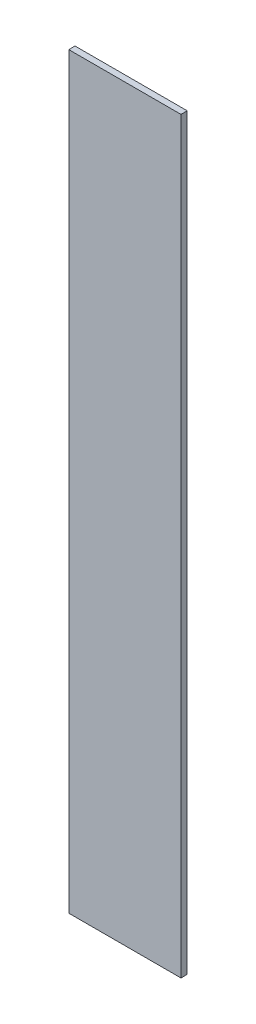
from build123d import *

# Parameters (mm, degrees)
SKETCH_1_W      = 90
SKETCH_1_H      = 600
EXTRUDE_1_DEPTH = 3
SKETCH_2_W      = 90
SKETCH_2_H      = 600
EXTRUDE_2_DEPTH = 2


with BuildPart() as part:
    # 草图1 → 凸台-拉伸1 (new body)
    with BuildSketch(Plane.XY):
        with Locations((45, 300)):
            Rectangle(SKETCH_1_W, SKETCH_1_H)
    extrude(amount=EXTRUDE_1_DEPTH)

    # 草图2 → 凸台-拉伸2 (add)
    with BuildSketch(Plane(origin=(0, 0, 0), x_dir=(-1, 0, 0), z_dir=(0, 0, -1))):
        with Locations((-45, 300)):
            Rectangle(SKETCH_2_W, SKETCH_2_H)
    extrude(amount=EXTRUDE_2_DEPTH)


solid = part.part
